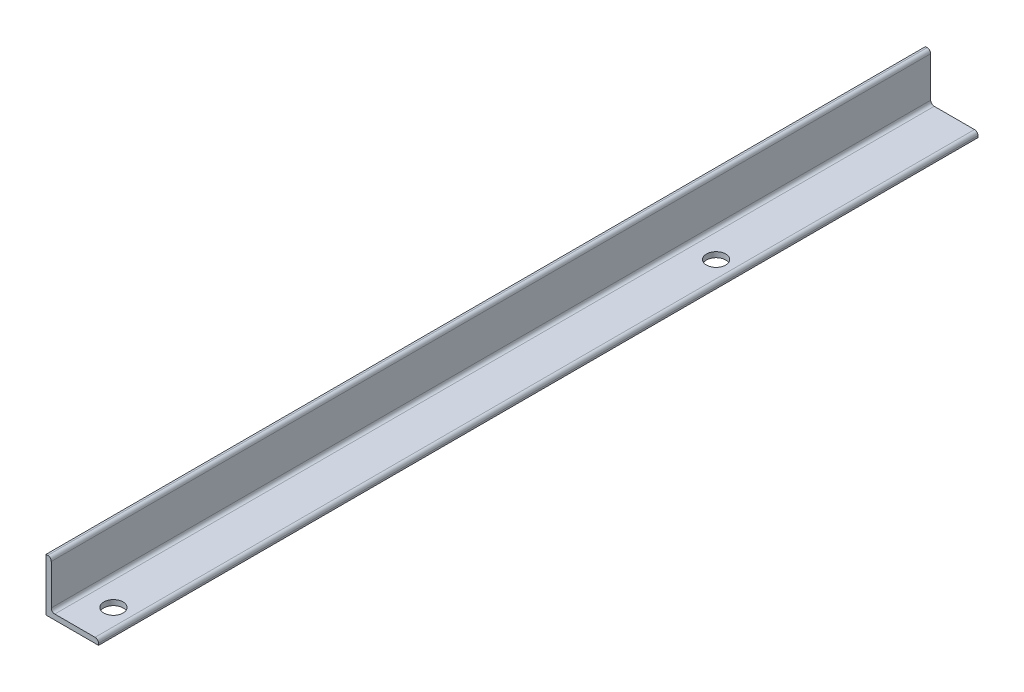
from build123d import *

# Parameters (mm, degrees)
BOSS_EXTRUDE1_DEPTH = 502
SKETCH2_R           = 5.5
CUT_EXTRUDE1_DEPTH  = 3
LPATTERN1_COUNT     = 2
LPATTERN1_PITCH     = 344


with BuildPart() as part:
    # Sketch1 → Boss-Extrude1 (new body)
    with BuildSketch(Plane.XY):
        with BuildLine():
            Line((0, 0), (30, 0))
            Line((30, 0), (30, 1))
            ThreePointArc((30, 1), (29.414213562, 2.414213562), (28, 3))
            Line((28, 3), (5, 3))
            ThreePointArc((5, 3), (3.585786438, 3.585786438), (3, 5))
            Line((3, 5), (3, 28))
            ThreePointArc((3, 28), (2.414213562, 29.414213562), (1, 30))
            Line((1, 30), (0, 30))
            Line((0, 30), (0, 0))
        make_face()
    extrude(amount=BOSS_EXTRUDE1_DEPTH)

    # Sketch2 → Cut-Extrude1 (cut)
    with BuildSketch(Plane.XZ):
        with Locations(Location((18.5, 482, 0), (0, 0, 270))):
            Circle(SKETCH2_R)
    cut_extrude1 = extrude(amount=-CUT_EXTRUDE1_DEPTH, mode=Mode.SUBTRACT)

    # LPattern1: Cut-Extrude1 ×2
    with Locations(*[(0, 0, -i * LPATTERN1_PITCH) for i in range(1, LPATTERN1_COUNT)]):
        add(cut_extrude1, mode=Mode.SUBTRACT)


solid = part.part
